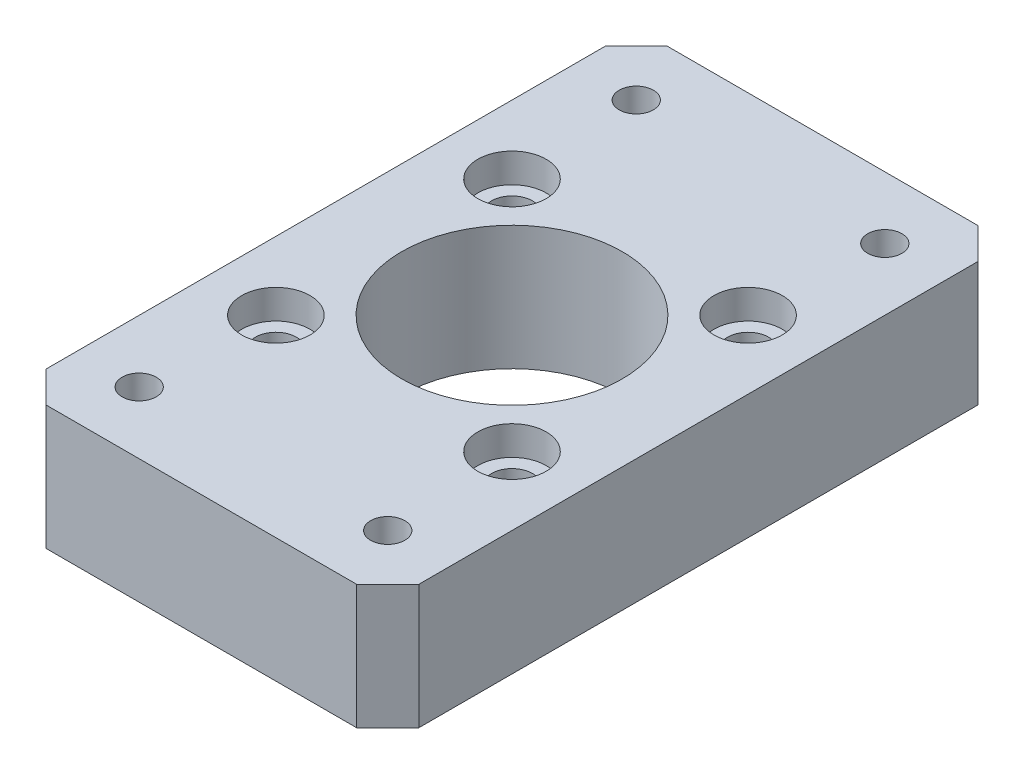
from build123d import *

# Parameters (mm, degrees)
SKETCH_1_W                  = 60
SKETCH_1_H                  = 100
EXTRUDE_1_DEPTH             = 20
SKETCH_2_R                  = 17.75
CUT_EXTRUDE_1_DEPTH         = 20
HOLE_WIZARD_1_D             = 6.6
HOLE_WIZARD_1_DEPTH         = 30
HOLE_WIZARD_1_CBORE_D       = 11
HOLE_WIZARD_1_CBORE_DEPTH   = 4.7
HOLE_WIZARD_1_TIP           = 1.982840043
CHAMFER_1_SIZE              = 5
HOLE_WIZARD_1_2_D           = 5.5
HOLE_WIZARD_1_2_DEPTH       = 30
HOLE_WIZARD_1_2_CBORE_D     = 10
HOLE_WIZARD_1_2_CBORE_DEPTH = 5.7
HOLE_WIZARD_1_2_TIP         = 1.652366702


with BuildPart() as part:
    # 草图1 → 凸台-拉伸1 (new body)
    with BuildSketch(Plane(origin=(0, 0, 0), x_dir=(1, 0, 0), z_dir=(0, 1, 0))):
        Rectangle(SKETCH_1_W, SKETCH_1_H)
    extrude(amount=EXTRUDE_1_DEPTH)

    # 草图2 → 切除-拉伸1 (cut)
    with BuildSketch(Plane(origin=(0, 20, 0), x_dir=(1, 0, 0), z_dir=(0, 1, 0))):
        with Locations(Location((0, 0, 0), (0, 0, 270))):
            Circle(SKETCH_2_R)
    extrude(amount=-CUT_EXTRUDE_1_DEPTH, mode=Mode.SUBTRACT)

    # Hole Wizard 1
    with Locations(Plane(origin=(0, 20, 0), x_dir=(1, 0, 0), z_dir=(0, 1, 0))):
        with Locations((19, 19), (19, -19), (-19, 19), (-19, -19)):
            CounterBoreHole(HOLE_WIZARD_1_D / 2, HOLE_WIZARD_1_CBORE_D / 2, HOLE_WIZARD_1_CBORE_DEPTH, depth=HOLE_WIZARD_1_DEPTH)
            with Locations((0, 0, -(HOLE_WIZARD_1_DEPTH + HOLE_WIZARD_1_TIP / 2))):  # 118° drill point
                Cone(0, HOLE_WIZARD_1_D / 2, HOLE_WIZARD_1_TIP, mode=Mode.SUBTRACT)

    # 倒角1
    chamfer_1_edges = [part.edges().sort_by_distance(p)[0] for p in [
        (30, 10, 50),
        (-30, 10, 50),
        (-30, 10, -50),
        (30, 10, -50),
    ]]
    chamfer(chamfer_1_edges, length=CHAMFER_1_SIZE)

    # Hole Wizard 1 2
    with Locations(Plane(origin=(0, 0, 0), x_dir=(-1, 0, 0), z_dir=(0, -1, 0))):
        with Locations((20, 40), (-20, 40), (20, -40), (-20, -40)):
            CounterBoreHole(HOLE_WIZARD_1_2_D / 2, HOLE_WIZARD_1_2_CBORE_D / 2, HOLE_WIZARD_1_2_CBORE_DEPTH, depth=HOLE_WIZARD_1_2_DEPTH)
            with Locations((0, 0, -(HOLE_WIZARD_1_2_DEPTH + HOLE_WIZARD_1_2_TIP / 2))):  # 118° drill point
                Cone(0, HOLE_WIZARD_1_2_D / 2, HOLE_WIZARD_1_2_TIP, mode=Mode.SUBTRACT)


solid = part.part
